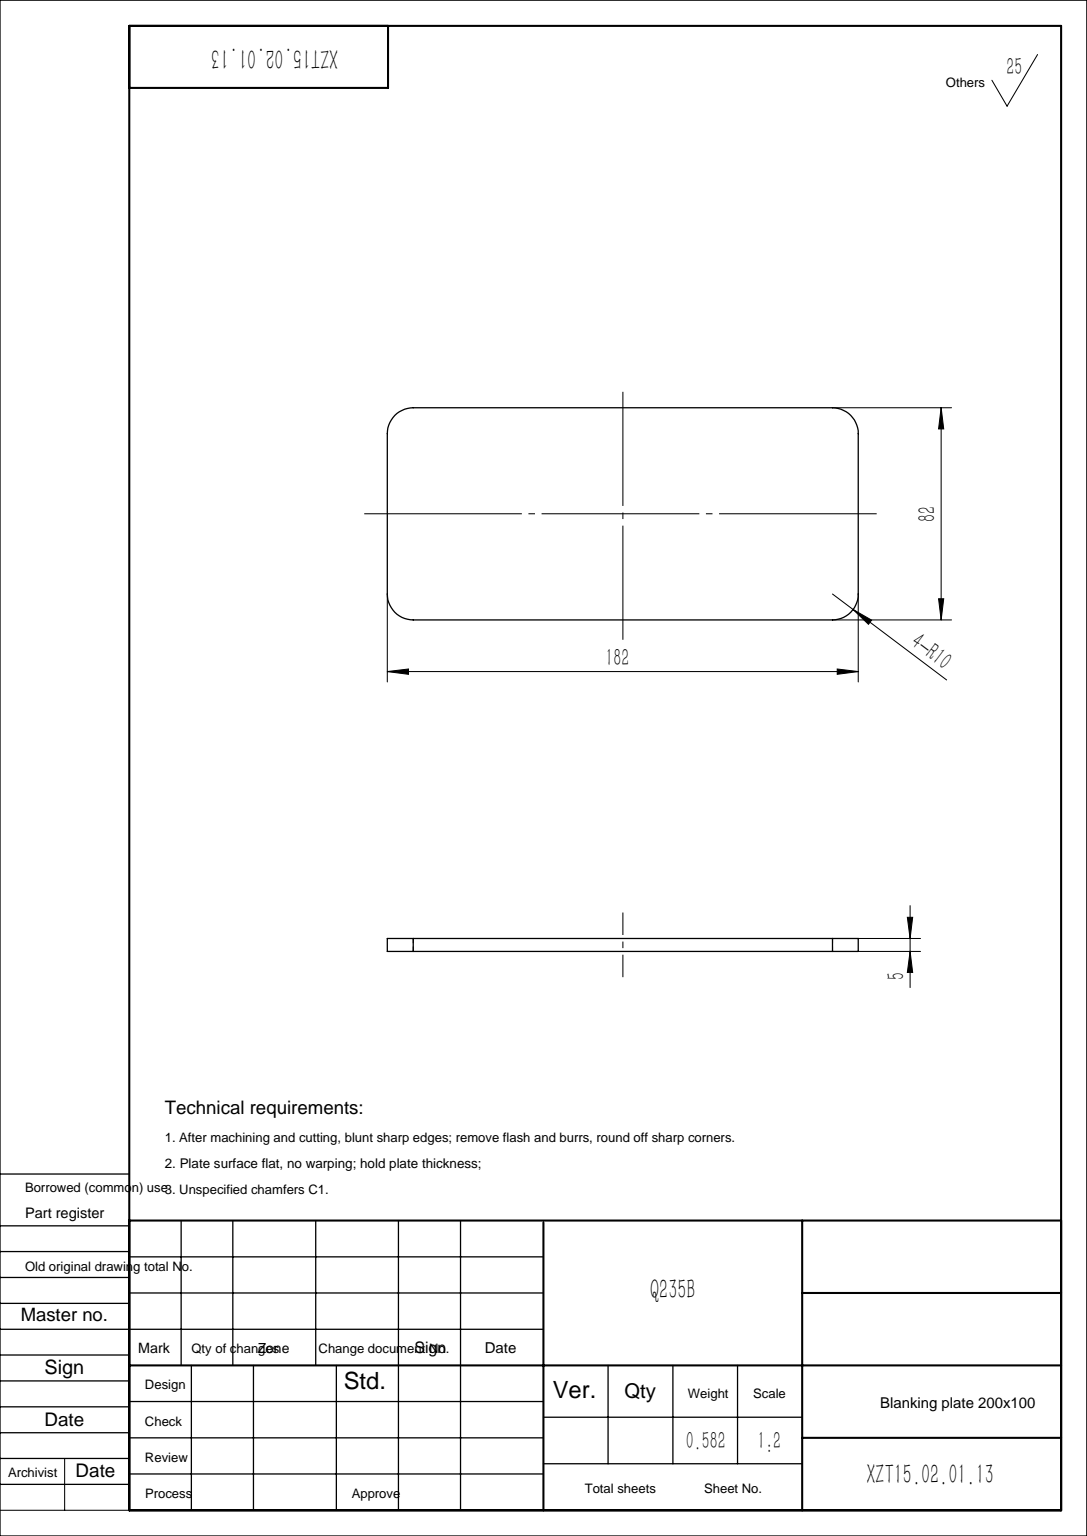
from build123d import *

# Parameters (mm, degrees)
SKETCH1_W           = 182
SKETCH1_H           = 82
BOSS_EXTRUDE1_DEPTH = 5
FILLET1_R           = 10


with BuildPart() as part:
    # Sketch1 → Boss-Extrude1 (new body)
    with BuildSketch(Plane(origin=(0, 0, 0), x_dir=(1, 0, 0), z_dir=(0, 1, 0))):
        Rectangle(SKETCH1_W, SKETCH1_H)
    extrude(amount=BOSS_EXTRUDE1_DEPTH)

    # Fillet1
    fillet1_edges = [part.edges().sort_by_distance(p)[0] for p in [
        (-91, 2.5, -41),
        (91, 2.5, -41),
        (91, 2.5, 41),
        (-91, 2.5, 41),
    ]]
    fillet(fillet1_edges, radius=FILLET1_R)


solid = part.part
